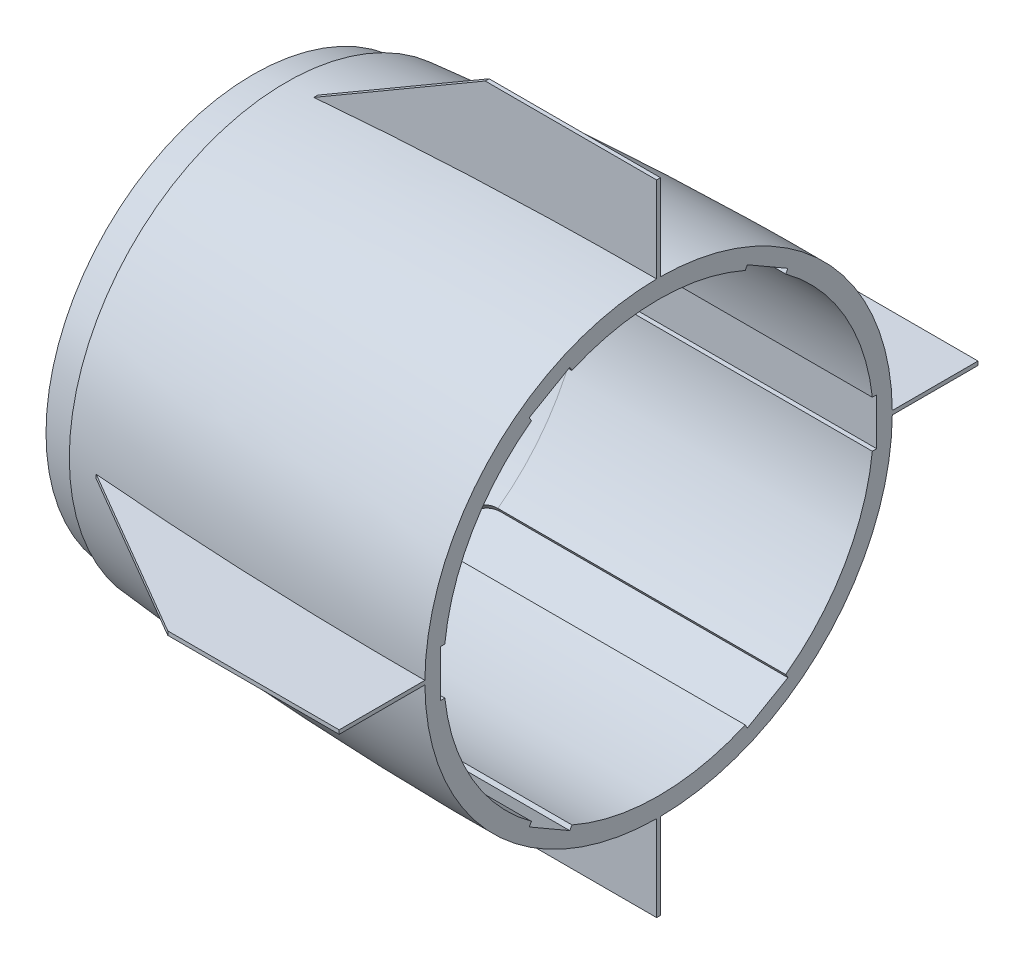
from build123d import *

# Parameters (mm, degrees)
CUT_EXTRUDE1_DEPTH      = 140
CIRPATTERN3_COUNT       = 6
BOSS_EXTRUDE2_DEPTH     = 1.25
CIRPATTERN5_COUNT       = 4
CUT_EXTRUDE2_DEPTH      = 140
CUT_EXTRUDE2_DEPTH_BACK = 160
SKETCH7_W               = 64.782558885
SKETCH7_H               = 314.406040355


with BuildPart() as part:
    # Sketch2 → Revolve3 (revolve)
    with BuildSketch(Plane.XY, mode=Mode.PRIVATE) as revolve3_sk:
        with BuildLine():
            add(Edge.make_bspline(
                [(450.637981389, 284.73247383), (547.084546243, 295.579175512), (643.913977944, 300.065614523), (733.25, 300)],
                knots=[0.61414211, 0.61414211, 0.61414211, 0.61414211, 1, 1, 1, 1], degree=3))
            Line((450.637981389, 284.73247383), (450.637981389, 280.422668446))
            add(Edge.make_bspline(
                [(429.254980688, 277.779677975), (436.406633809, 278.720600606), (443.534300709, 279.601597429), (450.637981389, 280.422668446)],
                knots=[0, 0, 0, 0, 0.176421293, 0.176421293, 0.176421293, 0.176421293], degree=3))
            Line((429.254980688, 277.779677975), (429.254980688, 273.462123081))
            Line((429.254980688, 273.462123081), (452.579811784, 276.562541937))
            Line((452.579811784, 276.562541937), (456.493793174, 281.086536072))
            add(Edge.make_bspline(
                [(456.493793174, 281.086536072), (503.218855637, 286.280028028), (548.555090765, 288.003752879)],
                knots=[0.224943096, 0.224943096, 0.224943096, 1, 1, 1], degree=2))
            Line((548.555090765, 288.003752879), (733.25, 288.003752879))
            Line((733.25, 288.003752879), (733.25, 300))
        make_face()
    revolve(revolve3_sk.sketch.rotate(Axis((0, 150, 0), (1, 0, 0)), 90), axis=Axis((0, 150, 0), (1, 0, 0)))

    # Sketch5 → Cut-Extrude1 (cut)
    with BuildSketch(Plane.XY):
        with BuildLine():
            Line((548.555090765, 165), (733.25, 165))
            Line((733.25, 165), (733.25, 135))
            Line((733.25, 135), (548.555090765, 135))
            ThreePointArc((548.555090765, 135), (533.555090765, 150), (548.555090765, 165))
        make_face()
    cut_extrude1 = extrude(amount=-CUT_EXTRUDE1_DEPTH, mode=Mode.SUBTRACT)

    # CirPattern3: Cut-Extrude1 ×6 about axis
    cirpattern3_axis = Axis((0, 150, 0), (1, 0, 0))
    for i in range(1, CIRPATTERN3_COUNT):
        add(cut_extrude1.rotate(cirpattern3_axis, i * 360 / CIRPATTERN3_COUNT), mode=Mode.SUBTRACT)

    # Sketch6 → Boss-Extrude2 (add, symmetric)
    with BuildSketch(Plane.XY):
        Polygon((733.25, 297.5), (733.25, 355), (623.25, 355), (513.25, 290.901062134), align=None)
    boss_extrude2 = extrude(amount=BOSS_EXTRUDE2_DEPTH, both=True)

    # CirPattern5: Boss-Extrude2 ×4 about axis
    cirpattern5_axis = Axis((0, 150, 0), (1, 0, 0))
    for i in range(1, CIRPATTERN5_COUNT):
        add(boss_extrude2.rotate(cirpattern5_axis, i * 360 / CIRPATTERN5_COUNT))

    # Sketch7 → Cut-Extrude2 (cut, two sides: drawn at the far end of the back side and taken through both)
    with BuildSketch(Plane.XY.offset(-CUT_EXTRUDE2_DEPTH_BACK)):
        with Locations((461.863701246, 144.750690011)):
            Rectangle(SKETCH7_W, SKETCH7_H)
    extrude(amount=CUT_EXTRUDE2_DEPTH + CUT_EXTRUDE2_DEPTH_BACK, mode=Mode.SUBTRACT)


with BuildPart() as body_2:
    # of the pieces the cut leaves, the one that is kept (cut_extrude2_keep)
    add(part.part.solids().sort_by_distance((494.254980688, 150, 139.21046037))[0])

    # Sketch8 → Revolve4 (revolve)
    with BuildSketch(Plane.XY, mode=Mode.PRIVATE) as revolve4_sk:
        with BuildLine():
            Line((500.01374771, 285.159819571), (500.01374771, 287.937524413))
            Line((500.01374771, 287.937524413), (494.254980688, 287.492248924))
            Line((494.254980688, 287.492248924), (494.254980688, 284.735755541))
            add(Edge.make_bspline(
                [(472.951688948, 282.852733411), (480.103342069, 283.793656042), (487.151300008, 283.914684525), (494.254980688, 284.735755541)],
                knots=[0, 0, 0, 0, 0.176421293, 0.176421293, 0.176421293, 0.176421293], degree=3))
            Line((472.951688948, 282.852733411), (472.951688948, 278.090955753))
            Line((472.951688948, 278.090955753), (495.811376327, 280.478482723))
            Line((495.811376327, 280.478482723), (500.01374771, 285.159819571))
        make_face()
    revolve(revolve4_sk.sketch.rotate(Axis((733.25, 150, 0), (-1, 0, 0)), 90), axis=Axis((733.25, 150, 0), (-1, 0, 0)))


solid = body_2.part
